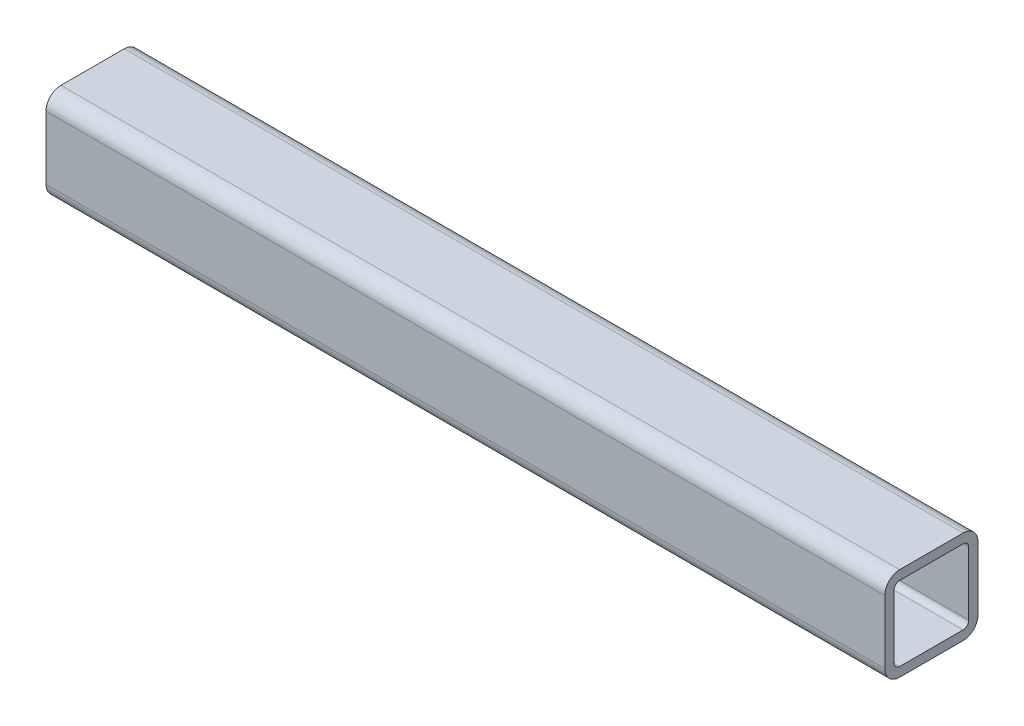
from build123d import *

# Parameters (mm, degrees)
COLD_FORMED_SQUARE_HOLLOW_SECTION_GB_T_6_DEPTH = 450


with BuildPart() as part:
    # Sketch1 → Cold-formed square hollow section GB/T 6728-2002 50 X 50 X 4(1) (new body)
    with BuildSketch(Plane.YZ.offset(-88.434077868)):
        with BuildLine():
            Line((-17, -25), (17, -25))
            ThreePointArc((17, -25), (22.656854249, -22.656854249), (25, -17))
            Line((25, -17), (25, 17))
            ThreePointArc((25, 17), (22.656854249, 22.656854249), (17, 25))
            Line((17, 25), (-17, 25))
            ThreePointArc((-17, 25), (-22.656854249, 22.656854249), (-25, 17))
            Line((-25, 17), (-25, -17))
            ThreePointArc((-25, -17), (-22.656854249, -22.656854249), (-17, -25))
        make_face()
        with BuildLine():
            Line((-17, -20), (17, -20))
            ThreePointArc((17, -20), (19.121320344, -19.121320344), (20, -17))
            Line((20, -17), (20, 17))
            ThreePointArc((20, 17), (19.121320344, 19.121320344), (17, 20))
            Line((17, 20), (-17, 20))
            ThreePointArc((-17, 20), (-19.121320344, 19.121320344), (-20, 17))
            Line((-20, 17), (-20, -17))
            ThreePointArc((-20, -17), (-19.121320344, -19.121320344), (-17, -20))
        make_face(mode=Mode.SUBTRACT)
    extrude(amount=COLD_FORMED_SQUARE_HOLLOW_SECTION_GB_T_6_DEPTH)


solid = part.part
